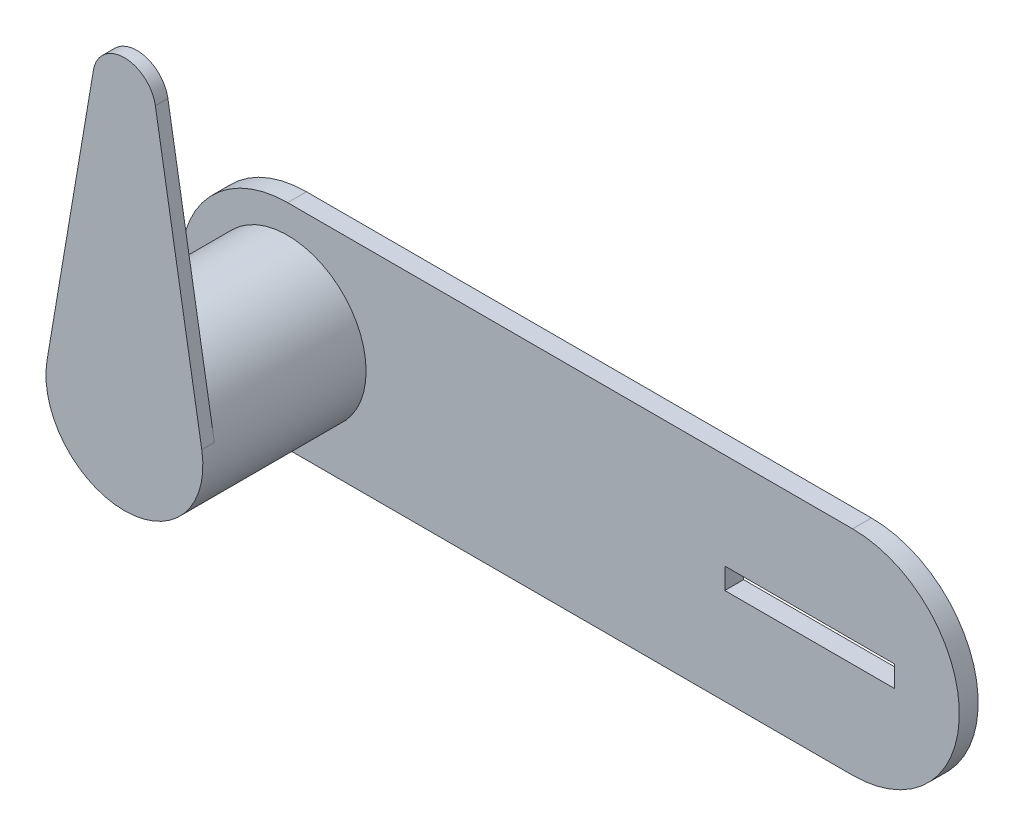
SolidWorks part; units mm, degrees
ref_plane "前视基准面" through (0, 0, 0) normal (0, 0, 1) x (1, 0, 0)
ref_plane "上视基准面" through (0, 0, 0) normal (0, 1, 0) x (1, 0, 0)
ref_plane "右视基准面" through (0, 0, 0) normal (1, 0, 0) x (0, 0, -1)
sketch "草图1" plane through (0, 0, 0) normal (0, 0, 1) x (1, 0, 0)
  line L0 (-45, 0) -> (45, 0) construction
  line L1 (-45, 17) -> (45, 17)
  line L2 (-45, -17) -> (45, -17)
  arc A0 (-45, 17) -> (-45, -17) centre (-45, 0) ccw
  arc A1 (45, -17) -> (45, 17) centre (45, 0) ccw
  point P2 (0, 0)
  dimension "D1" = 90
  dimension "D2" = 34
extrude "凸台-拉伸1" add sketch "草图1" along normal blind 3
sketch "草图2" plane through (0, 0, 0) normal (0, 0, -1) x (-1, 0, 0)
  line L1 (-51.6901, -1.6908) -> (-24.6373, -1.6908)
  line L2 (-51.6901, -1.6908) -> (-51.6901, 1.6908)
  line L3 (-51.6901, 1.6908) -> (-24.6373, 1.6908)
  line L4 (-24.6373, -1.6908) -> (-24.6373, 1.6908)
  line L5 (-51.6901, -1.6908) -> (-24.6373, 1.6908) construction
  line L6 (-51.6901, 1.6908) -> (-24.6373, -1.6908) construction
  point P0 (-38.1637, 0)
extrude "切除-拉伸1" cut sketch "草图2" against normal blind 3
sketch "草图3" plane through (0, 0, 3) normal (0, 0, 1) x (1, 0, 0)
  circle A0 centre (-45, 0) radius 12.5
  dimension "D1" = 25
extrude "凸台-拉伸2" add sketch "草图3" along normal blind 24
sketch "草图4" plane through (0, 0, 27) normal (0, 0, 1) x (1, 0, 0)
  line L0 (-45, 0) -> (-45, 45) construction
  line L1 (-57.3252, 2.0833) -> (-49.9301, 45.8333)
  line L2 (-40.0699, 45.8333) -> (-32.6748, 2.0833)
  arc A0 (-40.0699, 45.8333) -> (-49.9301, 45.8333) centre (-45, 45) ccw
  arc A1 (-57.3252, 2.0833) -> (-32.6748, 2.0833) centre (-45, 0) ccw
  dimension "D2" = 25
  dimension "D3" = 10
  dimension "D1" = 45
extrude "凸台-拉伸3" add sketch "草图4" along normal blind 2
